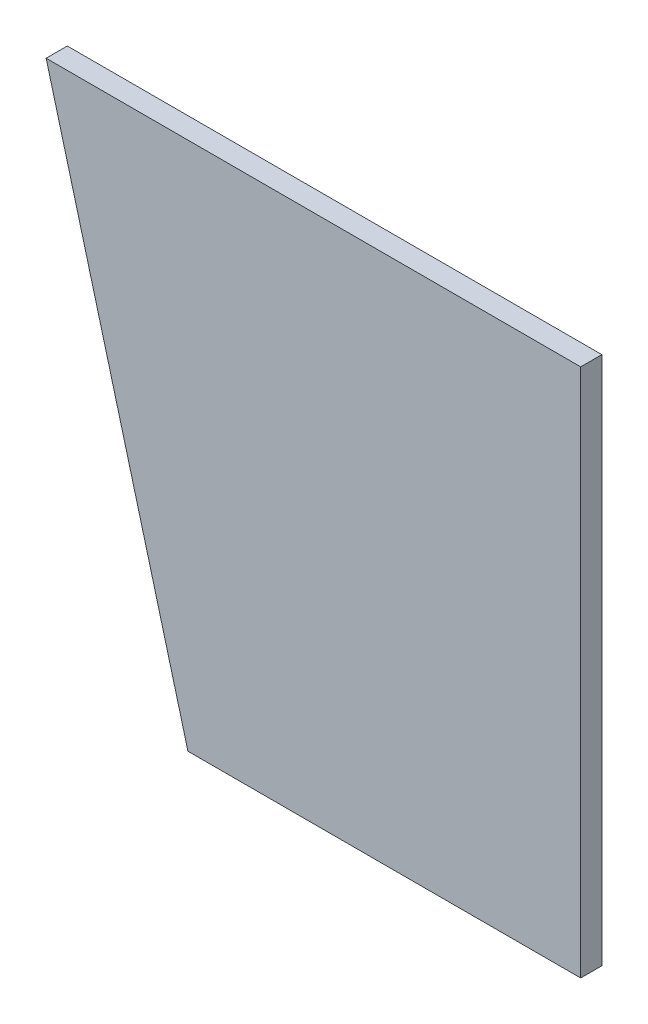
from build123d import *

# Parameters (mm, degrees)
EXTRUDE1_DEPTH = 6


with BuildPart() as part:
    # Sketch1 → Extrude1 (new, symmetric)
    with BuildSketch(Plane.XY):
        Polygon((-303, 0), (0, 0), (0, -300), (-222.615242271, -300), align=None)
    extrude(amount=EXTRUDE1_DEPTH, both=True)


solid = part.part
